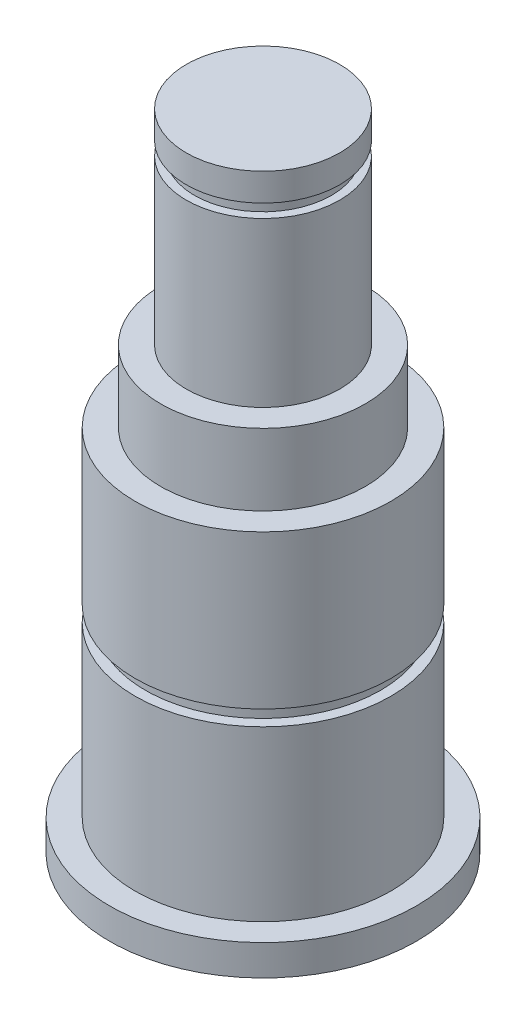
SolidWorks part; units mm, degrees
ref_plane "前视基准面" through (0, 0, 0) normal (0, 0, 1) x (1, 0, 0)
ref_plane "上视基准面" through (0, 0, 0) normal (0, 1, 0) x (1, 0, 0)
ref_plane "右视基准面" through (0, 0, 0) normal (1, 0, 0) x (0, 0, -1)
sketch "草图1" plane through (0, 0, 0) normal (0, 0, 1) x (1, 0, 0)
  line L0 (7.5, 65.7053) -> (0, 65.7053)
  line L1 (0, 65.7053) -> (0, 2.7053)
  line L2 (0, 2.7053) -> (15, 2.7053)
  line L3 (15, 2.7053) -> (15, 5.7053)
  line L4 (15, 5.7053) -> (12.5, 5.7053)
  line L5 (12.5, 5.7053) -> (12.5, 22.2053)
  line L6 (12.5, 22.2053) -> (11.5, 22.2053)
  line L7 (11.5, 22.2053) -> (11.5, 23.7053)
  line L8 (11.5, 23.7053) -> (12.5, 23.7053)
  line L9 (12.5, 23.7053) -> (12.5, 38.7053)
  line L10 (12.5, 38.7053) -> (10, 38.7053)
  line L11 (10, 38.7053) -> (10, 45.7053)
  line L12 (10, 45.7053) -> (7.5, 45.7053)
  line L13 (7.5, 45.7053) -> (7.5, 61.7053)
  line L14 (7.5, 61.7053) -> (6.7, 61.7053)
  line L15 (6.7, 61.7053) -> (6.7, 63.0053)
  line L16 (6.7, 63.0053) -> (7.5, 63.0053)
  line L17 (7.5, 63.0053) -> (7.5, 65.7053)
  line L18 (0, 65.7053) -> (0, 2.7053) construction
revolve "旋转1" add sketch "草图1" angle 360 about L18
